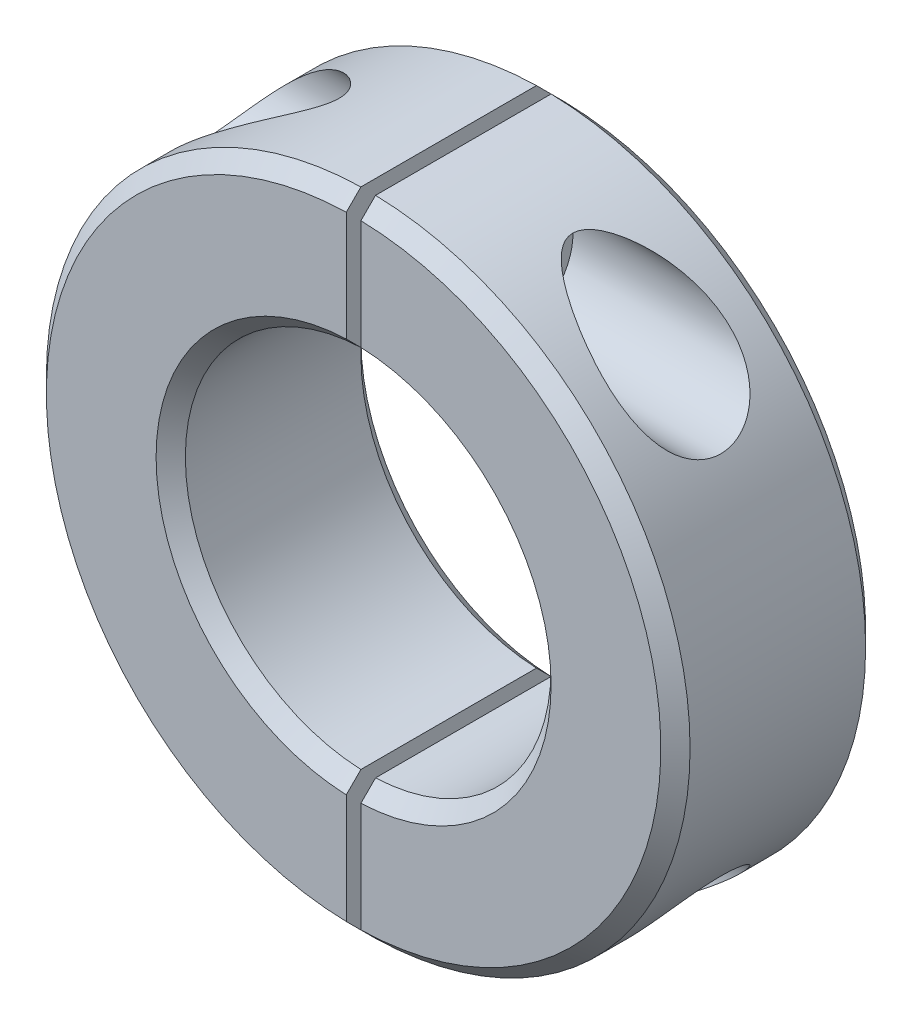
SolidWorks part; units mm, degrees
ref_plane "前视基准面" through (0, 0, 0) normal (0, 0, 1) x (1, 0, 0)
ref_plane "上视基准面" through (0, 0, 0) normal (0, 1, 0) x (1, 0, 0)
ref_plane "右视基准面" through (0, 0, 0) normal (1, 0, 0) x (0, 0, -1)
sketch "草图1" plane through (0, 0, 0) normal (0, 0, 1) x (1, 0, 0)
  line L0 (0, 22) -> (0, 12.5)
  line L1 (0, -12.5) -> (0, -22)
  arc A0 (0, -22) -> (0, 22) centre (0, 0) ccw
  arc A1 (0, -12.5) -> (0, 12.5) centre (0, 0) ccw
  dimension "D1" = 25
  dimension "D2" = 44
extrude "凸台-拉伸1" add sketch "草图1" along normal mid plane 14
chamfer "倒角1" distance 1 angle 45 4 edges at (22, 0, -7) (12.5, 0, -7) (12.5, 0, 7) (22, 0, 7)
sketch "草图2" plane through (0, 0, 7) normal (0, 0, 1) x (1, 0, 0)
  line L1 (-0.5, -37.6736) -> (0.5, -37.6736)
  line L2 (-0.5, -37.6736) -> (-0.5, 37.6736)
  line L3 (-0.5, 37.6736) -> (0.5, 37.6736)
  line L4 (0.5, -37.6736) -> (0.5, 37.6736)
  line L5 (-0.5, -37.6736) -> (0.5, 37.6736) construction
  line L6 (-0.5, 37.6736) -> (0.5, -37.6736) construction
  point P1 (0, 0)
  dimension "D1" = 1
extrude "切除-拉伸1" cut sketch "草图2" against normal through all
ref_plane "基准面1" through (4, 0, 0) normal (1, 0, 0) x (0, 0, -1)
sketch "草图3" plane through (4, 0, 0) normal (1, 0, 0) x (0, 0, -1)
  line L0 (0, 0) -> (0, -16.5) construction
  line L1 (0, 0) -> (21.3063, 0) construction
  circle A0 centre (0, -16.5) radius 4
  circle A1 centre (0, 16.5) radius 4
  dimension "D1" = 8
  dimension "D2" = 16.5
extrude "切除-拉伸2" cut sketch "草图3" along normal through all
sketch "草图4" plane through (4, 0, 0) normal (1, 0, 0) x (0, 0, -1)
  circle A0 centre (0, 16.5) radius 2.5
  circle A1 centre (0, -16.5) radius 2.5
  dimension "D1" = 5
  dimension "D2" = 5
extrude "切除-拉伸3" cut sketch "草图4" against normal up to next
mirror "镜向5" about plane through (0, 0, 0) normal (1, 0, 0) of bodies 111
